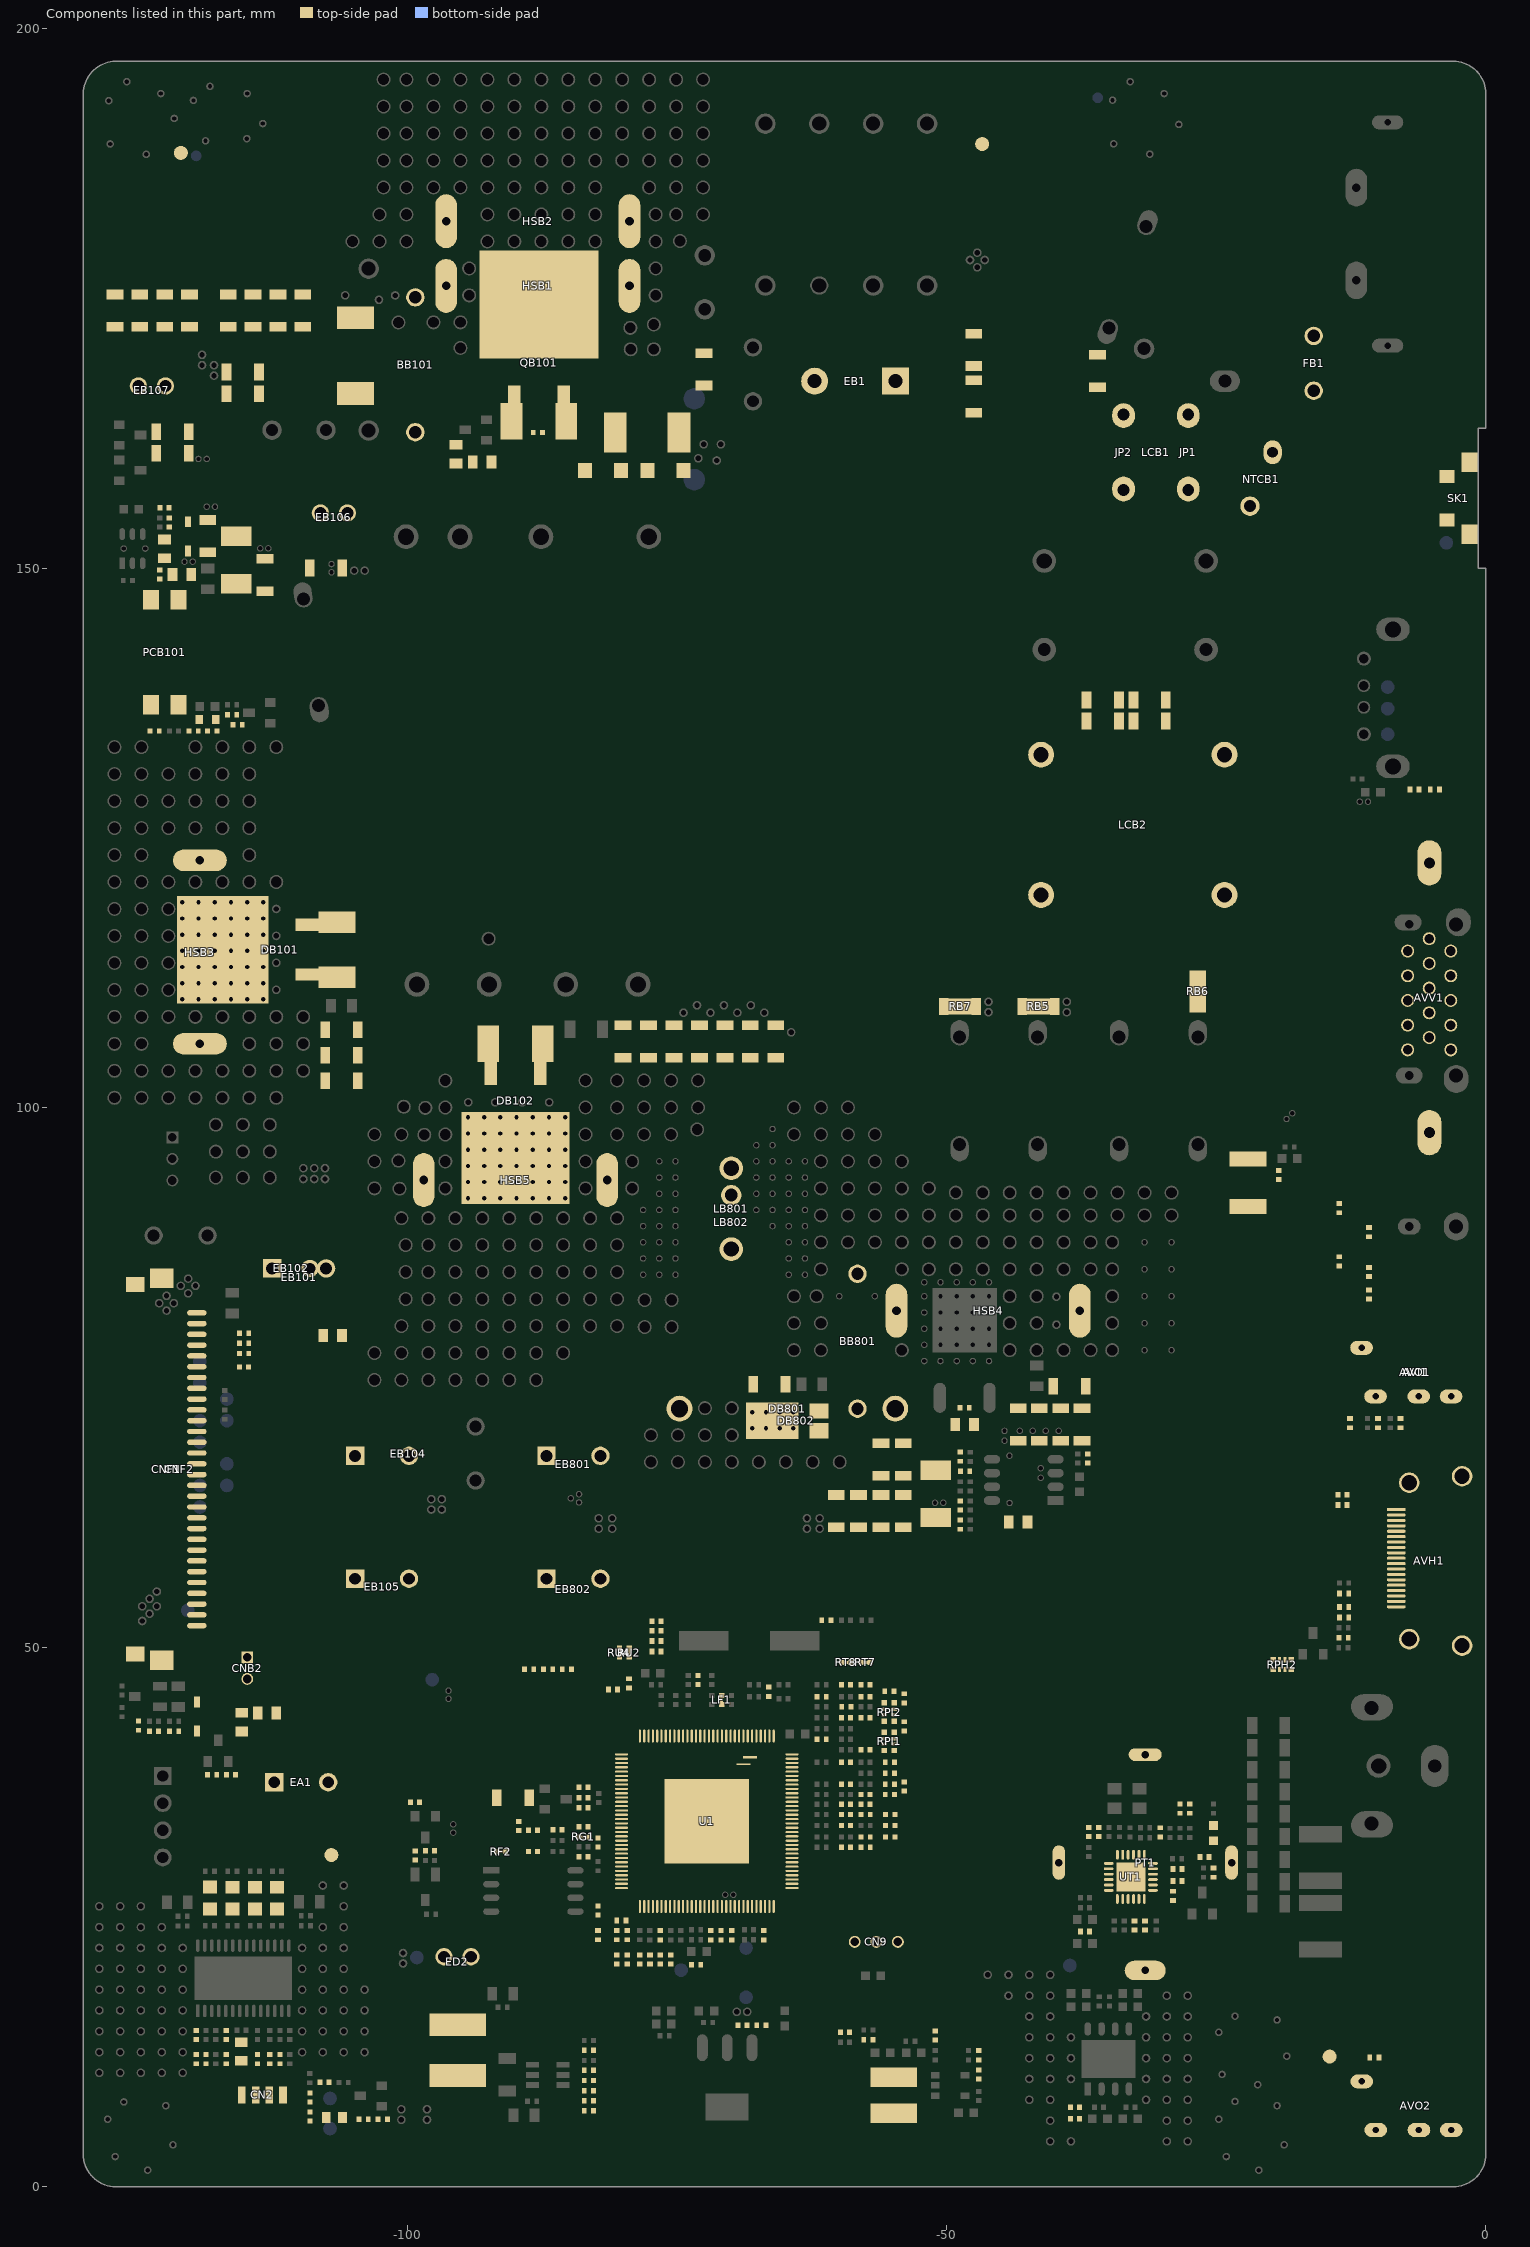
[diagram p0: the components of this part, seen from the top]
# Altium PCB MISC84438.PcbDoc (part 4 of 15)
Units mm, origin at the board's own origin, x right, y up, seen from the top; angles counter-clockwise.
Board outline 130 x 197 mm, 2 copper layers (TopLayer, BottomLayer), stack 1.571 mm thick; 574 components, 314 nets, 2636 pads, 811 vias.

## Footprints (in the part's own frame and the unit in brackets; to place one, negate y for a bottom-side part, rotate by r counter-clockwise, add the part's x,y. Pads: shape width x height; smd on the part's side, far side on the other; paste and mask are expansions set on the pad) (continued)
D2PAK3#2 [mm] "伟达电子；SFS1006G;增加TO-252兼容；160309"
  oval 2.794x1.143 smd: 1(5.542,-2.2) 3(5.542,2.4)
  rect 2.794x1.143 smd: 1(5.544,-2.2) 3(5.544,2.4)
  rect 3.4x2 smd paste-5 mask-5: 1(7.494,-2.44) 3(7.494,2.64)
  rect 10x11 smd paste-11 mask-11: 2(-3.356,0.1)
  rect 6x6 smd paste-10 mask-11: 2(-2.158,0.1)
  TopLayer pour cut-out: 3.373,2.4 6.497,2.4 6.497,-2.245 6.438,-2.54 6.271,-2.791 6.02,-2.958 5.725,-3.017 5.725,-3.017 5.725,-2.199 4.141,-2.199 4.141,-3.024 3.847,-2.966 3.598,-2.799 3.432,-2.55 3.373,-2.256 3.373,-2.256
  silkscreen extent -9.13,-5.69 4.84,5.89, body extent -6.91,-5.15 8.79,5.35, height 4.7
D3-H-20-2 [mm] "肖特基二极管;UF544~UF5408;15.04.14"
  round 2.6 on Top Overlay: 0(10,0) 1(-10,0)
  round 2.4 hole 1.6: A(-10,0) K(10,0)
  silkscreen extent -13,-3.15 13,3.15
DB15-HF-1 [mm] "兴万联电子：WLHD-051A"
  oval 4.4x2.4 on Top Overlay: 0(-12.5,5.227) 0(12.5,5.227)
  round 1.2 hole 0.9: 1(4.33,7.247) 2(2.04,7.247) 3(-0.25,7.247) 4(-2.54,7.247) 5(-4.83,7.247) 6(5.475,5.247) 7(3.185,5.247) 8(0.895,5.247) 9(-1.395,5.247) 10(-3.685,5.247) 11(4.33,3.247) 12(2.04,3.247) 13(-0.25,3.247) 14(-2.54,3.247) 15(-4.83,3.247)
  oval 4.2x2.2 hole 1 slot 3 at 0 deg: 16(-12.5,5.227) 17(12.5,5.227)
  round 1.5 on Top Overlay: 30(-4.83,3.247) 31(-2.54,3.247) 32(-0.25,3.247) 33(2.04,3.247) 34(4.33,3.247) 35(5.475,5.247) 36(3.185,5.247) 37(0.895,5.247) 38(-1.395,5.247) 39(-3.685,5.247) 40(-4.83,7.247) 41(-2.54,7.247) 42(-0.25,7.247) 43(2.04,7.247) 44(4.33,7.247)
  BottomLayer pour cut-out: -4.814,8.609 -4.814,5.885 -4.587,5.885 -4.443,5.742 -3.456,5.742 -3.175,5.461 -3.175,5.029 -3.454,4.75 -4.42,4.75 -4.56,4.609 -4.797,4.609 -4.83,4.576 -4.83,1.885 4.33,1.885 4.33,3.247 4.298,3.279 4.298,4.609 4.105,4.609 3.95,4.764 2.44,4.764 2.285,4.609 1.817,4.609 1.664,4.763 0.648,4.763 0.368,5.042 0.368,5.474 0.622,5.728 1.651,5.728 1.803,5.88 2.286,5.88 2.438,5.728 3.95,5.728 4.107,5.885 4.33,5.885 4.33,8.609
  silkscreen extent -15.59,0 15.59,9.48, body extent -16.75,-62.85 16.75,8.75, height 14.13
DIODE-S0402 [mm] "DVD上使用的ESD"
  rect 0.45x0.55 smd mask+0.051: A(-0.425,0) K(0.425,0)
  silkscreen extent -0.8,-0.43 0.91,0.43, body extent -0.5,-0.25 0.5,0.25, height 0.5
DIODE-S0603 [mil]
  rect 32x40 smd: A(-29.5,0) K(29.5,0)
  silkscreen extent -55,-30 63,30, body extent -31,-16 31,16, height 31
DIODE-S-2 [mm] "1N5819-SMA;170509去除兼容,20180607减少内距0.4mm以兼容SMAF"
  rect 1.8x2.8 smd: A(-2.2,0) K(2.2,0)
  silkscreen extent -3.5,-1.6 3.7,1.61, body extent -2.6,-1.4 2.6,1.4, height 1.91
DIODE-S-12 [mm] "Formosa MS ;BAV19WS THRU BAV21WS/PMEG2010BEA(高度为1.1mm)"
  rect 1x0.55 smd: A(1.35,0) K(-1.35,0)
  silkscreen extent -0.9,-0.67 0.9,0.67, body extent -1.35,-0.63 1.35,0.63, height 1
DIODE-S-13 [mm] "DIODES;SBR10U45SP5"
  rect 1.4x1.75 smd: 1(0.92,-2.925) 3(-0.92,-2.925)
  rect 3.36x4.86 smd: 2(0,1.4)
  silkscreen extent -2.03,-2.73 2.03,2.73, body extent -2.02,-3.3 2.02,3.3, height 1.15
DIODE-S-14 [mm] "ROHM;FSL14"
  rect 1.3x1.35 smd: A(1.675,0) K(-1.675,0)
  silkscreen extent -1.55,-1 1.55,1, body extent -1.95,-1 1.95,1, height 1.08
DIODE-SMC [mm] "SM320C~SM3200;DO-214AB;14-03-07"
  rect 2.1x3.4 smd: A(3.505,0) K(-3.505,0)
  silkscreen extent -3.55,-3.11 3.55,3.11, body extent -4.07,-3.11 4.07,3.11, height 2.5
EC(5*11)-V-2.5#1 [mm] "机插2.5间距"
  round 1.8 on Top Overlay: 0(-1.25,0) 0(1.25,0)
  round 0.5 on Keep-Out: 0(0,-0.787)
  round 1.6 hole 1.1: 1(-1.25,0) 2(1.25,0)
  BottomLayer lines w0.6: -1.64,-0.31 -1.67,-0.262 ; -1.25,0 -2.806,1.556 ; -0.94,0.39 -0.988,0.42 ; 0.94,-0.39 0.988,-0.42 1.25,-0.584 1.29,-0.608 1.743,-0.892 2.724,-1.504 2.806,-1.556 ; 1.25,0 1.29,-0.04 2.142,-0.892 2.806,-1.556 ; 1.64,0.31 1.67,0.262 2.391,-0.892 2.793,-1.536 2.806,-1.556 ; -2.806,1.556 -1.67,-0.262 ; -2.806,1.556 -0.988,0.42 ; -1.67,-0.262 -1.67,-0.262 ; -0.988,0.42 -0.988,0.42
  silkscreen extent -2.66,-2.67 3,2.67, body extent -2.48,-2.52 2.5,2.47, height 7
EC(5*11)-V-2.5#2 [mm] "机插2.5间距"
  round 1.8 on Top Overlay: 0(-1.25,0) 0(1.25,0)
  round 0.5 on Keep-Out: 0(0,-0.787)
  round 1.6 hole 1.1: 1(-1.25,0) 2(1.25,0)
  BottomLayer lines w0.6: -1.64,-0.31 -1.67,-0.262 ; -1.25,0 -2.806,1.556 ; -0.94,0.39 -0.988,0.42 ; 0.94,-0.39 0.988,-0.42 2.806,-1.556 ; 1.25,0 2.806,-1.556 ; 1.64,0.31 1.67,0.262 ; 1.67,0.262 2.806,-1.556 ; -2.806,1.556 -1.67,-0.262 ; -2.806,1.556 -0.988,0.42 ; -1.67,-0.262 -1.67,-0.262 ; -0.988,0.42 -0.988,0.42
  silkscreen extent -2.66,-2.67 3,2.67, body extent -2.48,-2.52 2.5,2.47, height 7
EC(6.3*11)-V-2.5 [mm] "机插2.5间距"
  round 0.5 on Keep-Out: 0(0,-0.889)
  round 1.6 hole 1.1: 1(-1.25,0) 2(1.25,0)
  round 1.8 on Top Overlay: 5(1.25,0) 6(-1.25,0)
  BottomLayer lines w0.6: -1.665,-0.275 -1.691,-0.225 -1.767,-0.076 -2.664,1.685 ; -1.25,0 -2.664,1.685 ; -0.907,0.361 -0.952,0.395 ; 0.907,-0.361 2.664,-1.685 ; 1.25,0 2.664,-1.685 ; 1.665,0.275 2.664,-1.685 ; -2.664,1.685 -0.952,0.395 ; -0.952,0.395 -0.952,0.395
  silkscreen extent -3.17,-3.17 3.51,3.17, body extent -3,-3 2.98,2.99, height 12
EC(8*11)-V-3.5 [mm]
  rect 1.6x1.6 hole 1: 1(-1.75,0)
  rect 1.8x1.8 on Top Overlay: 1(-1.75,0)
  round 1.8 on Top Overlay: 1(1.75,0)
  round 1.6 hole 1: 2(1.75,0)
  silkscreen extent -4.25,-4.25 4.45,4.25, body extent -3.98,-3.98 4.01,4.01, height 12.51
EC(10*12.5)-V-5#1 [mm] "机插5间距"
  round 0.5 on Keep-Out: 0(-0.75,0)
  rect 1.7x1.7 hole 1.1: 1(-2.5,0)
  rect 1.9x1.9 on Top Overlay: 1(-2.5,0)
  round 1.9 on Top Overlay: 1(2.5,0)
  round 1.7 hole 1.1: 2(2.5,0)
  BottomLayer lines w0.6: -2.89,-0.31 -4.056,1.556 ; -2.5,0 -4.056,1.556 ; -2.19,0.39 -4.056,1.556 ; 2.19,-0.39 4.056,-1.556 ; 2.5,0 4.056,-1.556 ; 2.89,0.31 4.056,-1.556
  silkscreen extent -5.2,-5.21 5.57,5.21, body extent -4.98,-4.99 5.01,4.99, height 12.01
EC(10*12.5)-V-5#2 [mm] "机插5间距"
  round 0.5 on Keep-Out: 0(-0.178,-1.651)
  rect 1.7x1.7 hole 1.1: 1(-2.5,0)
  rect 1.9x1.9 on Top Overlay: 1(-2.5,0)
  round 1.9 on Top Overlay: 1(2.5,0)
  round 1.7 hole 1.1: 2(2.5,0)
  BottomLayer lines w0.6: -2.89,-0.31 -2.92,-0.262 -4.056,1.556 ; -2.5,0 -4.056,1.556 ; -2.19,0.39 -2.238,0.42 -4.056,1.556 ; 2.19,-0.39 2.238,-0.42 ; 2.5,0 4.056,-1.556 ; 2.89,0.31 2.914,0.272 2.92,0.262 ; 2.238,-0.42 2.5,-0.584 4.056,-1.556 ; 2.238,-0.42 2.238,-0.42 ; 2.238,-0.42 2.238,-0.42 ; 2.92,0.262 4.056,-1.556 ; 2.92,0.262 2.92,0.262 ; 2.92,0.262 2.92,0.262
  silkscreen extent -5.2,-5.21 5.57,5.21, body extent -4.98,-4.99 5.01,4.99, height 12.01
EC(10*12.5)-V-5#3 [mm] "机插5间距"
  round 0.5 on Keep-Out: 0(7.315,0.419)
  rect 1.7x1.7 hole 1.1: 1(-2.5,0)
  rect 1.9x1.9 on Top Overlay: 1(-2.5,0)
  round 1.9 on Top Overlay: 1(2.5,0)
  round 1.7 hole 1.1: 2(2.5,0)
  BottomLayer lines w0.6: -2.92,-0.262 -2.89,-0.31 ; -2.92,-0.262 -2.928,-0.249 -2.967,-0.186 -2.995,-0.141 -3.109,0.041 -3.139,0.089 -4.056,1.556 ; -2.5,0 -2.524,0.024 -2.59,0.09 -2.63,0.13 -2.639,0.139 -2.641,0.141 -2.676,0.176 -2.926,0.426 -3.109,0.609 -3.139,0.639 -4.056,1.556 ; -2.19,0.39 -2.238,0.42 ; 2.19,-0.39 2.238,-0.42 ; 2.5,0 4.056,-1.556 ; 2.89,0.31 2.92,0.262 4.056,-1.556 ; -4.056,1.556 -3.139,0.983 -3.109,0.964 -2.676,0.694 -2.666,0.687 -2.639,0.67 -2.63,0.665 -2.524,0.599 -2.5,0.584 -2.322,0.472 -2.314,0.467 -2.251,0.428 -2.238,0.42 ; -2.238,0.42 -2.238,0.42 ; 2.238,-0.42 2.238,-0.42 ; 2.238,-0.42 2.5,-0.584 4.056,-1.556
  silkscreen extent -5.2,-5.21 5.57,5.21, body extent -4.98,-4.99 5.01,4.99, height 12.01
EC(10*12.5)-V-5#4 [mm] "机插5间距"
  round 0.5 on Keep-Out: 0(0.689,-1.452)
  rect 1.7x1.7 hole 1.1: 1(-2.5,0)
  rect 1.9x1.9 on Top Overlay: 1(-2.5,0)
  round 1.9 on Top Overlay: 1(2.5,0)
  round 1.7 hole 1.1: 2(2.5,0)
  BottomLayer lines w0.6: -2.92,-0.262 -2.89,-0.31 -2.89,-0.31 ; -2.92,-0.262 -2.926,-0.251 -3.16,0.123 -3.314,0.369 -3.524,0.705 -3.544,0.736 -3.716,1.011 -4.056,1.556 ; -2.5,0 -2.512,0.012 -2.524,0.024 -2.678,0.178 -3.092,0.591 -3.109,0.609 -3.16,0.66 -3.236,0.736 -3.287,0.787 -3.39,0.89 -4.056,1.556 ; -2.5,0.584 -2.285,0.449 -2.255,0.43 -2.238,0.42 ; -2.5,0.584 -2.524,0.599 -2.678,0.695 -2.81,0.777 -2.869,0.814 -3.044,0.924 -3.109,0.964 -3.16,0.996 -3.236,1.044 -4.056,1.556 ; -2.19,0.39 -2.197,0.394 -2.238,0.42 ; 2.19,-0.39 2.238,-0.42 4.056,-1.556 ; 2.5,0 4.056,-1.556 ; 2.89,0.31 2.92,0.262 2.92,0.262 ; -2.238,0.42 -2.238,0.42 ; -2.238,0.42 -2.238,0.42 ; 2.92,0.262 4.056,-1.556 ; 2.92,0.262 2.92,0.262
  silkscreen extent -5.2,-5.21 5.57,5.21, body extent -4.98,-4.99 5.01,4.99, height 12.01
EC(10*12.5)-V-5#5 [mm] "机插5间距"
  round 0.5 on Keep-Out: 0(-0.644,-1.549)
  rect 1.7x1.7 hole 1.1: 1(-2.5,0)
  rect 1.9x1.9 on Top Overlay: 1(-2.5,0)
  round 1.9 on Top Overlay: 1(2.5,0)
  round 1.7 hole 1.1: 2(2.5,0)
  BottomLayer lines w0.6: -2.89,-0.31 -2.92,-0.262 -3.084,0 -3.416,0.532 -3.759,1.081 -3.785,1.123 -4.056,1.556 ; -2.5,0 -3.416,0.916 -3.759,1.259 -3.785,1.285 -4.056,1.556 ; -2.19,0.39 -2.238,0.42 ; 2.19,-0.39 2.238,-0.42 ; 2.5,0 4.056,-1.556 ; 2.89,0.31 2.92,0.262 2.92,0.262 ; -4.056,1.556 -3.785,1.387 -3.759,1.37 -3.416,1.156 -2.5,0.584 -2.29,0.452 -2.238,0.42 ; -2.238,0.42 -2.238,0.42 ; 2.238,-0.42 2.238,-0.42 ; 2.238,-0.42 2.238,-0.42 ; 2.238,-0.42 2.5,-0.584 4.056,-1.556 ; 2.92,0.262 2.92,0.262 ; 2.92,0.262 4.056,-1.556
  silkscreen extent -5.2,-5.21 5.57,5.21, body extent -4.98,-4.99 5.01,4.99, height 12.01
EC(10*12.5)-V-5#6 [mm] "机插5间距"
  round 0.5 on Keep-Out: 0(2.01,-1.98)
  rect 1.7x1.7 hole 1.1: 1(-2.5,0)
  rect 1.9x1.9 on Top Overlay: 1(-2.5,0)
  round 1.9 on Top Overlay: 1(2.5,0)
  round 1.7 hole 1.1: 2(2.5,0)
  BottomLayer lines w0.6: -2.89,-0.31 -2.901,-0.292 -2.92,-0.262 -3.084,0 -3.089,0.008 -4.056,1.556 ; -2.5,0 -2.652,0.152 -2.798,0.298 -3.286,0.786 -4.056,1.556 ; -2.19,0.39 -2.222,0.41 -2.238,0.42 -2.5,0.584 -2.508,0.589 -2.652,0.679 -3.286,1.075 -3.52,1.221 -4.056,1.556 ; 2.19,-0.39 2.238,-0.42 ; 2.5,0 4.056,-1.556 ; 2.89,0.31 2.92,0.262 2.92,0.262 ; 2.238,-0.42 2.238,-0.42 ; 2.238,-0.42 2.238,-0.42 ; 2.238,-0.42 4.056,-1.556 ; 2.92,0.262 2.92,0.262 ; 2.92,0.262 4.056,-1.556
  silkscreen extent -5.2,-5.21 5.57,5.21, body extent -4.98,-4.99 5.01,4.99, height 12.01
EC(18*41)-H-7.5-1 [mm] "SAMXON  (18*40)，开槽"
  round 2.7 on Top Overlay: 1(-3.75,2.5)
  rect 2.5x2.5 hole 1.3: 1(3.75,2.5)
  rect 2.7x2.7 on Top Overlay: 1(3.75,2.5)
  round 2.5 hole 1.3: 2(-3.75,2.5)
  KeepOutLayer lines w0.127: -6.75,-46.5 -6.75,-2 6.75,-2 6.75,-46.5 -6.75,-46.5
  silkscreen extent -9.25,-46 9.25,2.5
FFC30H/1.0S-1 [mm] "禾昌兴业：196161-30041-3,  翻盖高度6.4mm"
  oval 0.5x1.8 smd: 1(-14.5,1.625) 2(-13.5,1.625) 3(-12.5,1.625) 4(-11.5,1.625) 5(-10.5,1.625) 6(-9.5,1.625) 7(-8.5,1.625) 8(-7.5,1.625) 9(-6.5,1.625) 10(-5.5,1.625) 11(-4.5,1.625) 12(-3.5,1.625) 13(-2.5,1.625) 14(-1.5,1.625) 15(-0.5,1.625) 16(0.5,1.625) 17(1.5,1.625) 18(2.5,1.625) 19(3.5,1.625) 20(4.5,1.625) 21(5.5,1.625) 22(6.5,1.625) 23(7.5,1.625) 24(8.5,1.625) 25(9.5,1.625) 26(10.5,1.625) 27(11.5,1.625) 28(12.5,1.625) 29(13.5,1.625) 30(14.5,1.625)
  rect 1.8x2.2 smd: 31(17.7,-1.625) 32(-17.7,-1.625)
  silkscreen extent -18.35,-5.13 18.35,4.23
FFC30H/1.0S-7 [mm] "CT,F10033FA030M1WL,掀盖翻开时最高5.24mm,0428_018"
  rect 0.4x1.2 smd mask+0.051: 1(-14.5,2.847)
  oval 0.4x1.2 smd mask+0.051: 2(-13.5,2.847) 3(-12.5,2.847) 4(-11.5,2.847) 5(-10.5,2.847) 6(-9.5,2.847) 7(-8.5,2.847) 8(-7.5,2.847) 9(-6.5,2.847) 10(-5.5,2.847) 11(-4.5,2.847) 12(-3.5,2.847) 13(-2.5,2.847) 14(-1.5,2.847) 15(-0.5,2.847) 16(0.5,2.847) 17(1.5,2.847) 18(2.5,2.847) 19(3.5,2.847) 20(4.5,2.847) 21(5.5,2.847) 22(6.5,2.847) 23(7.5,2.847) 24(8.5,2.847) 25(9.5,2.847) 26(10.5,2.847) 27(11.5,2.847) 28(12.5,2.847) 29(13.5,2.847) 30(14.5,2.847)
  rect 1.35x1.7 smd mask+0.051: 31(-17.125,-2.847) 32(17.125,-2.847)
  silkscreen extent -17.3,-4.55 17.3,5.2, body extent -17.21,-4.45 17.2,2.55, height 2.2
FUSE3.5A-S [mm] "FSMD 200R-2  Votage:8V"
  rect 1.4x3.45 smd: 1(-2.2,0) 2(2.2,0)
  silkscreen extent -3.4,-2 3.4,2, body extent -2.36,-1.71 2.36,1.71, height 1.2
"FUSE8.5*4-V-5(T3.15AL 250V~)" [mm] "SMT1315AP/2010T1A250VA1(编带/华德)"
  round 1.7 hole 1.15: 1(2.54,0) 2(-2.54,0)
  round 1.9 on Top Overlay: 4(2.54,0) 5(-2.54,0)
  BottomLayer lines w1: -2.312,0.271 -2.338,0.289 -3.977,1.437 ; 2.811,0.228 2.829,0.202 2.844,0.182 2.971,0 3.977,-1.437 ; -2.54,0 -3.977,1.437 ; 2.54,0 2.562,-0.022 3.977,-1.437 ; -2.811,-0.228 -2.829,-0.202 -2.971,0 -3.977,1.437 ; 2.312,-0.271 2.338,-0.289 2.367,-0.31 3.977,-1.437
  silkscreen extent -4.3,-2.1 4.3,2.1, body extent -4.3,-2.1 4.3,2.1, height 8.5
GND#1 [mm] "导通线"
  rect 0.66x0.203 smd paste-0.45 mask-0.45: JP_1K(-0.32,0) JP_2K(0.32,0)
GND#2 [mm] "导通线"
  rect 0.66x0.152 smd paste-0.45 mask-0.45: JP_1K(-0.32,0) JP_2K(0.32,0)
HDMI-HS-11 [mm] "客供；R-S151U-162;垫高；15.06.11(18.08.31 更新钢网）"
  rect 0.28x1.75 smd: 1(4.75,7.7)
  oval 0.28x1.75 smd: 2(4.25,7.7) 3(3.75,7.7) 4(3.25,7.7) 5(2.75,7.7) 6(2.25,7.7) 7(1.75,7.7) 8(1.25,7.7) 9(0.75,7.7) 10(0.25,7.7) 11(-0.25,7.7) 12(-0.75,7.7) 13(-1.25,7.7) 14(-1.75,7.7) 15(-2.25,7.7) 16(-2.75,7.7) 17(-3.25,7.7) 18(-3.75,7.7) 19(-4.25,7.7)
  rect 3x4 on Top Paste: 4(-7.45,2.3) 4(-7.25,6.6) 4(7.25,6.6) 4(7.45,2.3)
  round 1.9 hole 1.4 mask+0.076: 20(-7.25,6.5) 21(-7.85,1.6) 22(7.85,1.6) 23(7.25,6.5)
  silkscreen extent -7.5,-0.02 7.5,8.41, body extent -10.25,-81.2 10.25,9.06, height 12.13
"Heat-Shrinkable Tube" [mm] "收缩前壁厚0.3+-0.05，收缩后壁厚0.6+-0.1"
  round 0.3 on Mech2: 0(0,0)
"High Voltage" [mm]
  silkscreen extent -0.53,-1.52 0.43,1.27
HOT [mm]
HS038 [mm]
  oval 2x5 hole 0.8 slot 4 at 90 deg: 1(-8.5,0) 2(8.5,0)
  oval 2.2x5.2 on Top Overlay: 1(-8.5,0) 1(8.5,0)
  silkscreen extent -8.5,-2.5 8.5,2.5, body extent -8.86,-2.5 8.64,2.5, height 11.25
HS(14*14*6) [mm] "14×14×06-THD;14.10.21"
  silkscreen extent -7.1,-7.1 7.1,10.57
JP7.0#1 [mm] "双面板跳线,17.06.09"
  oval 2.3x2.1 hole 1.1 copper offset 0.1,0: 1(-3.5,0)
  oval 2.5x2.3 on Top Overlay: 1(-3.5,0) 1(3.5,0)
  oval 2.3x2.1 hole 1.1 copper offset -0.1,0: 2(3.5,0)
  BottomLayer lines w0.6: -3.392,0.68 -3.29,0.647 ; 3.392,0.68 3.29,0.647 1.3,0 ; -3.5,0 -1.3,0 ; 3.5,0 1.3,0 ; -3.392,-0.68 -3.29,-0.647 ; 3.392,-0.68 3.29,-0.647 1.3,0 ; -3.29,0.647 -1.3,0 ; -3.29,0.647 -3.29,0.647 ; -1.3,0 -3.29,-0.647 ; -3.29,-0.647 -3.29,-0.647
  silkscreen extent -2.61,-0.49 2.6,0.49
JP7.0#2 [mm] "双面板跳线,17.06.09"
  oval 2.3x2.1 hole 1.1 copper offset 0.1,0: 1(-3.5,0)
  oval 2.5x2.3 on Top Overlay: 1(-3.5,0) 1(3.5,0)
  oval 2.3x2.1 hole 1.1 copper offset -0.1,0: 2(3.5,0)
  BottomLayer lines w0.6: -3.392,0.68 -3.29,0.647 ; 3.392,0.68 1.3,0 ; -3.5,0 -1.3,0 ; 3.5,0 1.3,0 ; -3.392,-0.68 -3.29,-0.647 ; 3.392,-0.68 1.3,0 ; -3.29,0.647 -1.3,0 ; -3.29,0.647 -3.29,0.647 ; -1.3,0 -3.29,-0.647 ; -3.29,-0.647 -3.29,-0.647
  silkscreen extent -2.61,-0.49 2.6,0.49
KEY-HS-5 [mm] "春生电子（KFC-011SB-H3.5-EP）/TS06PW0-G35F(YF); 1  . 2脚为信号和地脚"
  rect 1.2x1.4 smd: 1(2,2.9) 2(-2,2.9)
  rect 1.8x1.6 smd: 3(-3.35,0.767) 4(3.35,0.767)
  round 0.85 on Keep-Out: ""(-1.15,1.3) ""(1.15,1.3)
  silkscreen extent -3.5,-0.7 3.5,2.8
L0402 [mm] "电感"
  rect 0.45x0.55 smd mask+0.076: 1(-0.425,0) 2(0.425,0)
  silkscreen extent -0.8,-0.42 0.8,0.43, body extent -0.5,-0.25 0.5,0.25, height 0.5
L0603 [mm] "片式磁珠、电感、ESD"
  rect 0.813x0.8 smd mask+0.076: 1(-0.706,0) 2(0.706,0)
  silkscreen extent -1.27,-0.55 1.27,0.55, body extent -0.8,-0.4 0.8,0.4, height 0.8
L0805 [mm] "片式磁珠、电感"
  rect 1.2x1.3 smd: 1(-1.016,0) 2(1.016,0)
  silkscreen extent -1.92,-0.95 1.92,0.95, body extent -1,-0.62 1,0.63, height 1.25
L(4.5*3.5)-S [mm] "SMD4532-6R8M-023"
  rect 1.8x4.3 smd: 1(-1.65,0) 2(1.65,0)
  TopLayer pour cut-out: -0.76,2.15 0.796,2.15 0.796,2.141 0.796,-2.149 -0.756,-2.149 -0.756,-2.15
  silkscreen extent -2.83,-2.44 3.3,2.44
L(6.0*4.5)-S [mm] "SWPA6045S4R7MT(Sunlord) :功率电感;161103更新焊盘大小"
  rect 2.1x5.2 smd paste-6: 1(-2.35,0) 2(2.35,0)
  TopLayer pour cut-out: -1.282,2.552 1.294,2.543 1.297,-2.547 -1.311,-2.549
  silkscreen extent -3.16,-3.15 3.9,3.15, body extent -3,-3 3,3, height 4.5
L(13.5*15.5)-V-5 [mm] "深圳秀益达；SA-A048-036-A SPK1214RBL-680K；14.11.19"
  round 1.9 hole 1.2 mask+0.076: 1(-2.5,0) 2(2.5,0)
  round 2.1 on Top Overlay mask+0.076: 3(-2.5,0) 4(2.5,0)
  silkscreen extent -6.75,-6.75 6.75,6.75, body extent -6.72,-6.73 6.72,6.75, height 15.5
L/LC2/15*14.5-V7.5 [mm] "SYDR1212-L003-YMX"
  round 2.2 hole 1.4: 1(-3.75,0) 2(3.75,0)
  round 2.4 on Top Overlay: 1(-3.75,0) 1(3.75,0)
  silkscreen extent -7.25,-7.25 7.25,7.25
L/LC4/12.8*10-V-6*7 [mm] "CK,SYT09-L230uA,18.05.23"
  round 1.7 hole 1 mask+0.051: 1(-3,-3.5) 2(3,-3.5) 3(3,3.5) 4(-3,3.5)
  round 1.9 on Top Overlay: 5(-3,3.5) 6(-3,-3.5) 7(3,-3.5) 8(3,3.5)
  silkscreen extent -6.4,-5 6.4,5
L/LC4/21*17-H-17*13 [mm] "CH,SQ1614-10.5mH,1206_2018"
  round 2.6 on Top Overlay mask+0.076: 0(-8.5,6.5) 0(-8.5,-6.5) 0(8.5,6.5) 0(8.5,-6.5)
  round 2.4 hole 1.4 mask+0.076: 1(-8.5,-6.5) 2(8.5,-6.5) 3(8.5,6.5) 4(-8.5,6.5)
  silkscreen extent -10.5,-8.5 10.5,8.5, body extent -10.5,-8.5 10.5,8.5, height 13.99
LB/3.5*6*12.5#1 [mm] "Φ3.5×6.0×0.65mm(编带/秀益达)"
  round 1.7 hole 1.15: 1(-6.25,0) 2(6.25,0)
  round 1.9 on Top Overlay: 35(-6.25,0) 36(6.25,0)
  BottomLayer lines w0.6: 6.185,-0.532 6.121,-0.516 ; -6.185,-0.532 -6.121,-0.516 -4.138,-0.022 ; 6.25,0 5.05,0 4.05,0 ; -6.25,0 -6.181,0 -6.046,0 -5.91,0 -4.05,0 ; 6.185,0.532 6.121,0.516 5.811,0.439 5.382,0.332 4.05,0 ; -6.185,0.532 -6.121,0.516 -6.046,0.498 -5.778,0.431 -4.05,0 ; 6.121,-0.516 5.942,-0.472 4.05,0 ; 6.121,-0.516 6.121,-0.516 ; -4.138,-0.022 -4.091,-0.01 -4.05,0 ; -4.138,-0.022 -4.138,-0.022
  silkscreen extent -5.6,-1.85 5.65,1.85, body extent -6.57,-1.75 6.58,1.75, height 3.5
LB/3.5*6*12.5#2 [mm] "Φ3.5×6.0×0.65mm(编带/秀益达)"
  round 1.7 hole 1.15: 1(-6.25,0) 2(6.25,0)
  round 1.9 on Top Overlay: 35(-6.25,0) 36(6.25,0)
  BottomLayer lines w0.6: 6.185,-0.532 6.121,-0.516 5.933,-0.469 4.05,0 ; -6.185,-0.532 -6.121,-0.516 -4.374,-0.081 -4.05,0 ; 6.25,0 5.828,0 4.05,0 ; -6.25,0 -4.172,0 -4.05,0 ; 6.185,0.532 6.121,0.516 4.05,0 ; -6.185,0.532 -6.121,0.516 -4.05,0
  silkscreen extent -5.6,-1.85 5.65,1.85, body extent -6.57,-1.75 6.58,1.75, height 3.5
Manufacture_Info [mm]
  round 0.3 on Mech2: 0(0,0)
MARK [mm] "SMD 使用"
  round 1.3 smd paste+0 mask+0.65: 0(0,0)
  TopLayer circle w0.254: c0,0 r1.444
  TopLayer pour cut-out: -1.3,0 -1.201,-0.497 -0.919,-0.919 -0.497,-1.201 0,-1.3 0,-1.3 0.497,-1.201 0.919,-0.919 1.201,-0.497 1.3,0 1.3,0 1.201,0.497 0.919,0.919 0.497,1.201 0,1.3 0,1.3 -0.497,1.201 -0.919,0.919 -1.201,0.497 -1.3,0
"NO DOLBY-SILK" [mm]
  silkscreen extent -0.4,-4.5 36.6,5
NTC(10*5)-V5 [mm] "热敏电阻 SCK152R58MSY  (为勤电子）;161022更新椭圆孔"
  round 1.8 hole 1.1: 1(-2.5,1.05)
  round 2 on Top Overlay: 2(-2.5,1.05)
  oval 2.2x1.7 hole 1 slot 1.5 at 0 deg: 2(2.5,-1.05)
  oval 2.4x1.9 on Top Overlay: 3(2.5,-1.05)
  silkscreen extent -5.77,-2.5 5.77,2.5, body extent -5.75,-2 5.75,2, height 13.75
OC4-S-1 [mm] "巨路国际；肖特基LTV-817S-TA-B"
  rect 1.5x1.8 smd: 1(-1.27,-4.88) 2(1.27,-4.88) 3(1.27,4.88) 4(-1.27,4.88)
  silkscreen extent -3.17,-5.35 2.55,3.5, body extent -2.3,-5.08 2.3,5.08, height 3.88
PCB_NAME [mm]
  round 0.3 on Mech2: 0(0,0)
PCB_TIME [mm]
  round 0.3 on Mech2: 0(0,0)
PHONE-HD-43 [mm] "乐友；CK3-3.5-03C;160624"
  oval 1.5x2.3 on Top Overlay: 0(-2.25,10.2) 0(-2.25,3.2) 0(-2.25,6.2) 0(2.25,11.5)
  round 1.1 on Keep-Out: 0(0,8.5) 0(0,1.5)
  oval 1.3x2.1 hole 0.6 slot 1.4 at 90 deg: 1(2.25,11.5) 2(-2.25,10.2) 3(-2.25,3.2) 4(-2.25,6.2)
  silkscreen extent -3.1,0 3.1,12.7
QFN24/0.5-3 [mm] "R620D(Rafael Micro)，修改EPAD焊盘/CY8C4014LQI-422(0.6mm)"
  oval 0.9x0.26 smd: 1(-2.05,1.25) 2(-2.05,0.75) 3(-2.05,0.25) 4(-2.05,-0.25) 5(-2.05,-0.75) 6(-2.05,-1.25) 13(2.05,-1.25) 14(2.05,-0.75) 15(2.05,-0.25) 16(2.05,0.25) 17(2.05,0.75) 18(2.05,1.25)
  oval 0.26x0.9 smd: 7(-1.25,-2.05) 8(-0.75,-2.05) 9(-0.25,-2.05) 10(0.25,-2.05) 11(0.75,-2.05) 12(1.25,-2.05) 19(1.25,2.05) 20(0.75,2.05) 21(0.25,2.05) 22(-0.25,2.05) 23(-0.75,2.05) 24(-1.25,2.05)
  rect 2.7x2.7 smd paste-2 mask-2: 25(0,0)
  silkscreen extent -3.33,-3.33 3.21,3.35, body extent -2.08,-2.07 2.07,2.07, height 1
QFP128/0.4-5 [mm] "IT9076/IT9072"
  rect 0.203x1.2 smd: 1(-6.2,-7.9)
  oval 0.203x1.2 smd: 2(-5.8,-7.9) 3(-5.4,-7.9) 4(-5,-7.9) 5(-4.6,-7.9) 6(-4.2,-7.9) 7(-3.8,-7.9) 8(-3.4,-7.9) 9(-3,-7.9) 10(-2.6,-7.9) 11(-2.2,-7.9) 12(-1.8,-7.9) 13(-1.4,-7.9) 14(-1,-7.9) 15(-0.6,-7.9) 16(-0.2,-7.9) 17(0.2,-7.9) 18(0.6,-7.9) 19(1,-7.9) 20(1.4,-7.9) 21(1.8,-7.9) 22(2.2,-7.9) 23(2.6,-7.9) 24(3,-7.9) 25(3.4,-7.9) 26(3.8,-7.9) 27(4.2,-7.9) 28(4.6,-7.9) 29(5,-7.9) 30(5.4,-7.9) 31(5.8,-7.9) 32(6.2,-7.9) 65(6.2,7.9) 66(5.8,7.9) 67(5.4,7.9) 68(5,7.9) 69(4.6,7.9) 70(4.2,7.9) 71(3.8,7.9) 72(3.4,7.9) 73(3,7.9) 74(2.6,7.9) 75(2.2,7.9) 76(1.8,7.9) 77(1.4,7.9) 78(1,7.9) 79(0.6,7.9) 80(0.2,7.9) 81(-0.2,7.9) 82(-0.6,7.9) 83(-1,7.9) 84(-1.4,7.9) 85(-1.8,7.9) 86(-2.2,7.9) 87(-2.6,7.9) 88(-3,7.9) 89(-3.4,7.9) 90(-3.8,7.9) 91(-4.2,7.9) 92(-4.6,7.9) 93(-5,7.9) 94(-5.4,7.9) 95(-5.8,7.9) 96(-6.2,7.9)
  oct 2x2 on Top Paste paste-1: 9(-2.3,-2.3) 9(-2.3,0) 9(-2.3,2.3) 9(0,2.3) 9(0,0) 9(0,-2.3) 9(2.3,-2.3) 9(2.3,0) 9(2.3,2.3)
  oct 2x2 on Top Solder paste-1: 9(-2.3,-2.3) 9(-2.3,0) 9(-2.3,2.3) 9(0,2.3) 9(0,0) 9(0,-2.3) 9(2.3,-2.3) 9(2.3,0) 9(2.3,2.3)
  oval 1.2x0.203 smd: 33(7.9,-6.2) 34(7.9,-5.8) 35(7.9,-5.4) 36(7.9,-5) 37(7.9,-4.6) 38(7.9,-4.2) 39(7.9,-3.8) 40(7.9,-3.4) 41(7.9,-3) 42(7.9,-2.6) 43(7.9,-2.2) 44(7.9,-1.8) 45(7.9,-1.4) 46(7.9,-1) 47(7.9,-0.6) 48(7.9,-0.2) 49(7.9,0.2) 50(7.9,0.6) 51(7.9,1) 52(7.9,1.4) 53(7.9,1.8) 54(7.9,2.2) 55(7.9,2.6) 56(7.9,3) 57(7.9,3.4) 58(7.9,3.8) 59(7.9,4.2) 60(7.9,4.6) 61(7.9,5) 62(7.9,5.4) 63(7.9,5.8) 64(7.9,6.2) 97(-7.9,6.2) 98(-7.9,5.8) 99(-7.9,5.4) 100(-7.9,5) 101(-7.9,4.6) 102(-7.9,4.2) 103(-7.9,3.8) 104(-7.9,3.4) 105(-7.9,3) 106(-7.9,2.6) 107(-7.9,2.2) 108(-7.9,1.8) 109(-7.9,1.4) 110(-7.9,1) 111(-7.9,0.6) 112(-7.9,0.2) 113(-7.9,-0.2) 114(-7.9,-0.6) 115(-7.9,-1) 116(-7.9,-1.4) 117(-7.9,-1.8) 118(-7.9,-2.2) 119(-7.9,-2.6) 120(-7.9,-3) 121(-7.9,-3.4) 122(-7.9,-3.8) 123(-7.9,-4.2) 124(-7.9,-4.6) 125(-7.9,-5) 126(-7.9,-5.4) 127(-7.9,-5.8) 128(-7.9,-6.2)
  rect 7.8x7.8 smd paste-5 mask-5: 129(0,0)
  silkscreen extent -9.34,-9.88 9.68,9.39, body extent -8,-8 8,8, height 1.61
R0402 [mm] "片式电阻"
  rect 0.45x0.5 smd mask+0.076: 1(-0.425,0) 2(0.425,0)
  silkscreen extent -0.8,-0.4 0.8,0.4, body extent -0.5,-0.25 0.5,0.25, height 0.5
R0402SC [mm]
  rect 0.45x0.5 smd mask+0.076: 1(-0.425,0) 2(0.425,0)
  rect 0.42x0.25 smd paste-0.5 mask-0.5: 3(0,0)
  silkscreen extent -0.8,-0.4 0.8,0.4
R0603 [mm] "贴片电阻"
  rect 0.7x0.8 smd mask+0.076: 1(-0.756,0) 2(0.756,0)
  silkscreen extent -1.25,-0.54 1.25,0.54, body extent -0.8,-0.4 0.8,0.4, height 0.8
R0805 [mm] "贴片电阻"
  rect 0.9x1.2 smd mask+0.076: 1(-0.866,0) 2(0.866,0)
  silkscreen extent -1.47,-0.75 1.47,0.75, body extent -1,-0.62 1,0.63, height 0.5
R1206 [mm] "贴片电阻"
  rect 0.9x1.55 smd mask+0.076: 1(-1.5,0) 2(1.5,0)
  silkscreen extent -2.1,-0.93 2.1,0.93, body extent -1.6,-0.8 1.6,0.8, height 0.55
R1206SC [mm] "贴片电阻"
  rect 0.9x1.55 smd mask+0.076: 1(-1.5,0) 2(1.5,0)
  rect 2.7x1.5 smd paste-2.7 mask-2.7: 3(0,0)
  silkscreen extent -2.1,-0.93 2.1,0.93, body extent -1.6,-0.8 1.6,0.8, height 0.55
R2512-1 [mm] "PSA;Size 2512 2W;16.01.20(17.06.19修改焊盘大小，增强爬锡，解决浮高问题）"
  rect 2.1x3.7 smd: 1(-2.95,0) 2(2.95,0)
  silkscreen extent -3.3,-2 3.3,2, body extent -3.25,-1.65 3.25,1.65, height 0.75
RA0402 [mm] "排阻"
  rect 0.5x0.5 smd mask+0.076: 1(-0.45,0.85) 2(0.45,0.85) 7(-0.45,-0.85) 8(0.45,-0.85)
  rect 0.5x0.3 smd mask+0.076: 3(-0.45,0.25) 4(0.45,0.25) 5(-0.45,-0.25) 6(0.45,-0.25)
  silkscreen extent -0.85,-1.27 0.85,1.27, body extent -0.51,-1 0.51,1, height 0.35
REMOTE-HS-1 [mm] "vishay;HS75438D;侧卧贴；14.09.03"
  rect 0.7x1.6 smd mask+0.076: 1(-1.905,2.275) 2(-0.635,2.275) 3(0.635,2.275) 4(1.905,2.275)
  silkscreen extent -3.47,-0.7 3.47,2.65
SHIELD(16*20*6) [mm] "屏蔽罩：用于与高频头分离的做法"
  oval 2.1x4.1 on Top Overlay: 0(-8,10) 0(8,10)
  oval 4.1x2.1 on Top Overlay: 0(0,0) 0(0,20)
  oval 3.8x1.8 hole 0.7 slot 2.7 at 0 deg: 1(0,0)
  oval 1.165x3.19 / inner oval 1.8x3.8 / far side oval 1.8x3.8 hole 0.7 slot 2.7 at 90 deg: 2(8,10) 4(-8,10)
  oval 3.063x1.165 / inner oval 3.8x1.8 / far side oval 3.8x1.8 hole 0.7 slot 2.7 at 0 deg: 3(0,20)
  silkscreen extent -9,-1 9,21, body extent -8.57,-0.15 8.57,20.15, height 6
"Silica gel-20" [mm] "硅胶"
  silkscreen extent -3,-10 3,10
SIP2/2.0D-1 [mm] "捷仕泰/铭锋达"
  rect 1.3x1.3 on Top Overlay: 0(-1,0)
  round 1.3 on Top Overlay: 0(1,0)
  rect 1.1x1.1 hole 0.8: 1(-1,0)
  round 1.1 hole 0.8: 2(1,0)
  silkscreen extent -3,-3.2 3,1.8, body extent -3,-3.2 3,1.8, height 6
SIP3/2.0D-3 [mm] "捷仕泰   A2004-03-A1MA-P,插线高度11mm"
  rect 1.5x1.5 on Top Overlay: 0(-2,0)
  round 1.5 on Top Overlay: 0(0,0) 0(2,0)
  round 1.1 / inner rect 1.1x1.1 / far side rect 1.1x1.1 hole 0.8: 1(-2,0)
  round 1.1 hole 0.8: 2(0,0) 3(2,0)
  silkscreen extent -4,-2.13 4,3.07